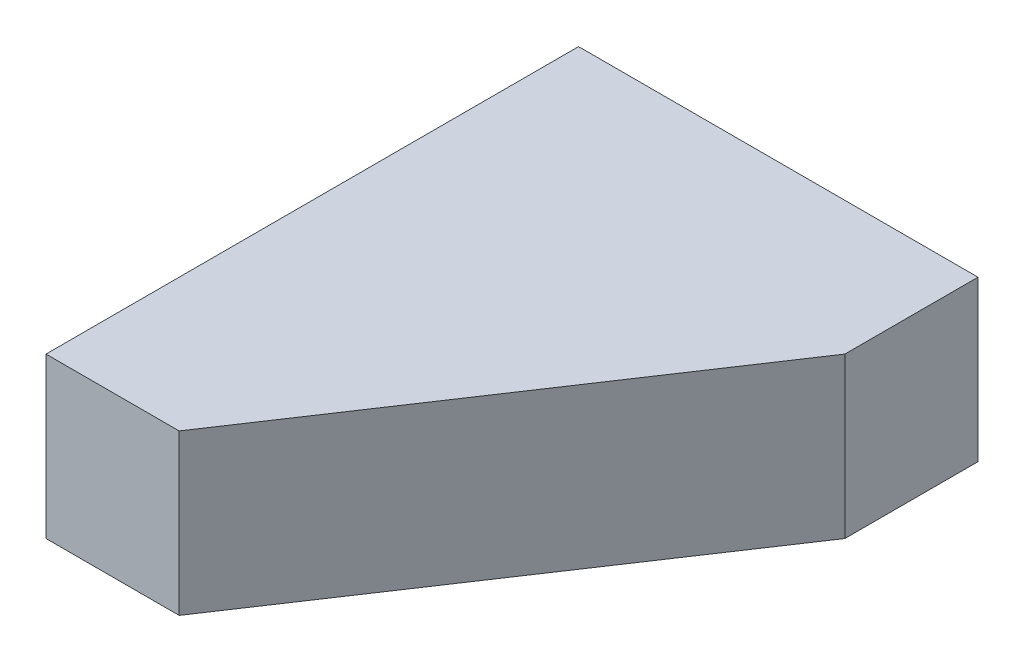
SolidWorks part; units mm, degrees
material "普通碳钢"
ref_plane "Front Plane" through (0, 0, 0) normal (0, 0, 1) x (1, 0, 0)
ref_plane "Top Plane" through (0, 0, 0) normal (0, 1, 0) x (1, 0, 0)
ref_plane "Right Plane" through (0, 0, 0) normal (1, 0, 0) x (0, 0, -1)
sketch "Sketch1" plane through (0, 0, 0) normal (0, 1, 0) x (1, 0, 0)
  line L0 (-15, -20) -> (-5, -20)
  line L1 (15, 20) -> (-15, 20)
  line L2 (-15, 20) -> (-15, -20)
  line L3 (15, 20) -> (15, 10)
  line L4 (15, 10) -> (-5, -20)
  point P3 (0, 20)
  point P5 (-15, 0)
  dimension "D1" = 40
  dimension "D2" = 30
  dimension "D3" = 10
  dimension "D4" = 10
extrude "Extrude1" add sketch "Sketch1" along normal mid plane 12
